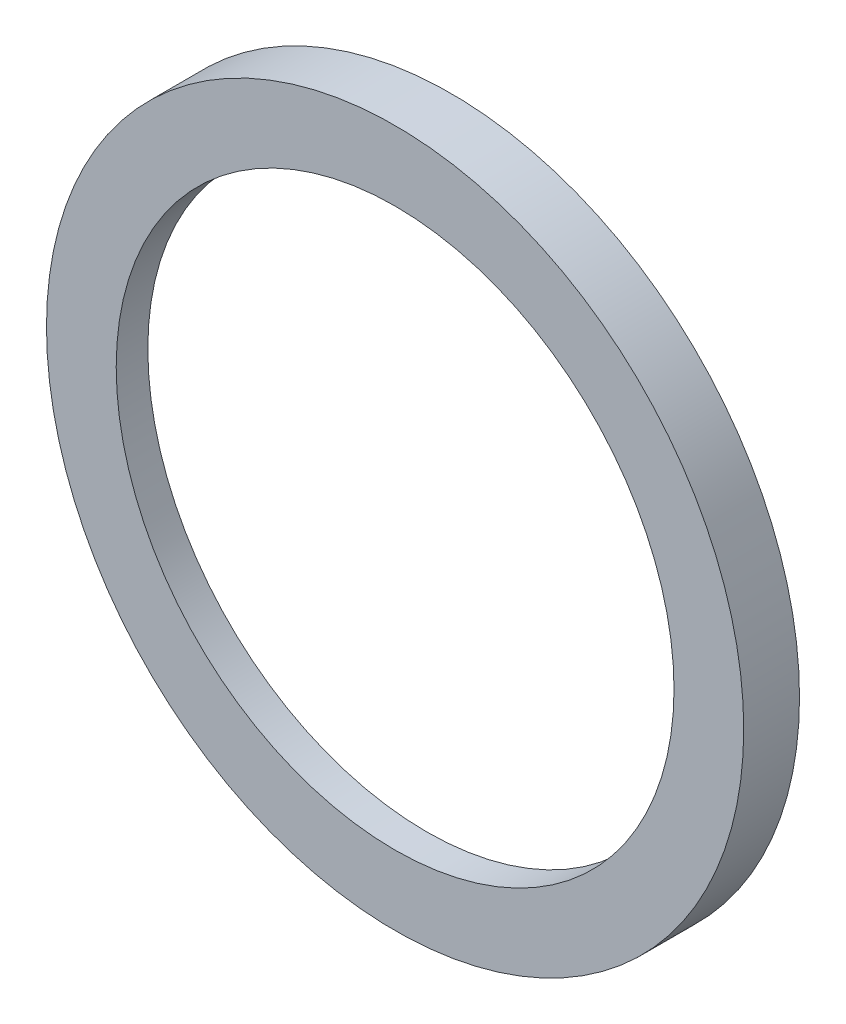
from build123d import *

# Parameters (mm, degrees)
M8_TAPPED_HOLE1_D     = 6.8
M8_TAPPED_HOLE1_DEPTH = 10.957073895
M8_TAPPED_HOLE1_TIP   = 2.042926105


with BuildPart() as part:
    # Sketch1 → Revolve1 (revolve)
    with BuildSketch(Plane(origin=(0, 0, 0), x_dir=(0, 0, -1), z_dir=(1, 0, 0)), mode=Mode.PRIVATE) as revolve1_sk:
        Polygon((0, 150), (0, 187.5), (30, 187.5), (30, 176), (17, 176), (17, 150), align=None)
    revolve(revolve1_sk.sketch.rotate(Axis((0, 0, 0), (0, 0, -1)), 90), axis=Axis((0, 0, 0), (0, 0, -1)))

    # M8 Tapped Hole1
    with Locations(Plane(origin=(0, 0, -17), x_dir=(-1, 0, 0), z_dir=(0, 0, -1))):
        with Locations((0, 162.5), (95.515103498, 131.465261586), (154.546683898, 50.215261586), (154.546683898, -50.215261586), (95.515103498, -131.465261586), (0, -162.5), (-95.515103498, -131.465261586), (-154.546683898, -50.215261586), (-154.546683898, 50.215261586), (-95.515103498, 131.465261586)):
            Hole(M8_TAPPED_HOLE1_D / 2, depth=M8_TAPPED_HOLE1_DEPTH)
            with Locations((0, 0, -(M8_TAPPED_HOLE1_DEPTH + M8_TAPPED_HOLE1_TIP / 2))):  # 118° drill point
                Cone(0, M8_TAPPED_HOLE1_D / 2, M8_TAPPED_HOLE1_TIP, mode=Mode.SUBTRACT)


solid = part.part
